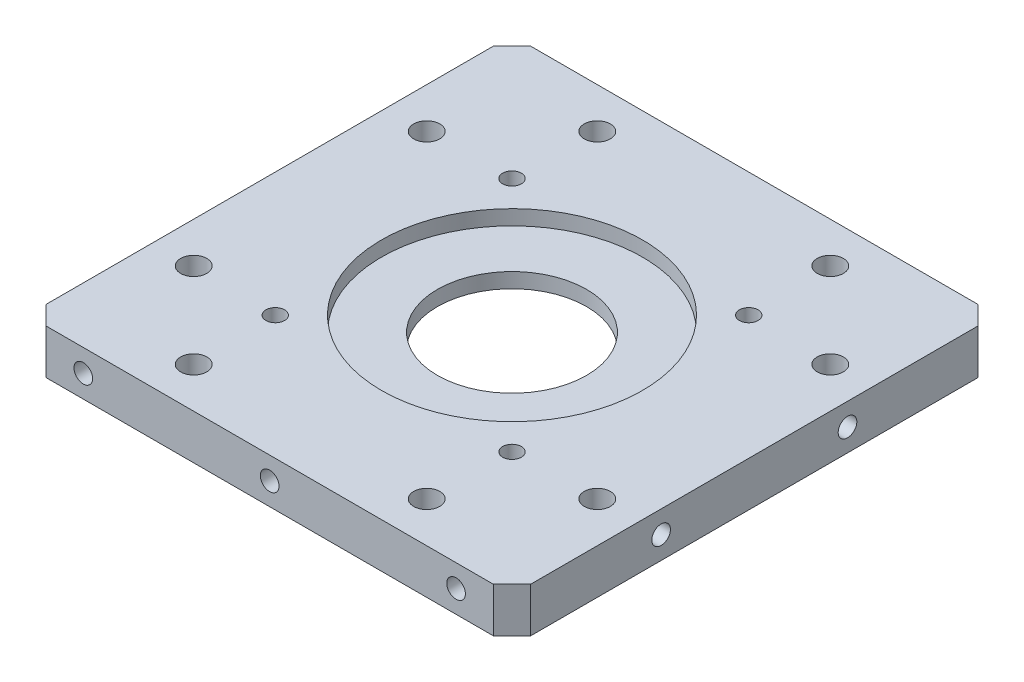
from build123d import *

# Parameters (mm, degrees)
SKETCH_1_W             = 130
SKETCH_1_H             = 130
EXTRUDE_1_DEPTH        = 12
SKETCH_2_R             = 20
CUT_EXTRUDE_1_DEPTH    = 93.703829479
HOLE_WIZARD_M6_1_D     = 7
SKETCH_5_R             = 35
CUT_EXTRUDE_2_DEPTH    = 4
SKETCH_6_R             = 45
CUT_EXTRUDE_3_DEPTH    = 4
HOLE_WIZARD_M6_1_2_D   = 5
HOLE_WIZARD_M6_2_D     = 5
HOLE_WIZARD_M6_2_DEPTH = 15
HOLE_WIZARD_M6_2_TIP   = 1.502151548
HOLE_WIZARD_M6_3_D     = 5
HOLE_WIZARD_M6_3_DEPTH = 15
HOLE_WIZARD_M6_3_TIP   = 1.502151548
HOLE_WIZARD_M6_4_D     = 5
HOLE_WIZARD_M6_4_DEPTH = 15
HOLE_WIZARD_M6_4_TIP   = 1.502151548
HOLE_WIZARD_M6_5_D     = 5
HOLE_WIZARD_M6_5_DEPTH = 15
HOLE_WIZARD_M6_5_TIP   = 1.502151548
CHAMFER_1_SIZE         = 5


with BuildPart() as part:
    # 草图1 → 凸台-拉伸1 (new body)
    with BuildSketch(Plane(origin=(0, 0, 0), x_dir=(1, 0, 0), z_dir=(0, 1, 0))):
        Rectangle(SKETCH_1_W, SKETCH_1_H)
    extrude(amount=EXTRUDE_1_DEPTH)

    # 草图2 → 切除-拉伸1 (cut, through all)
    with BuildSketch(Plane(origin=(0, 12, 0), x_dir=(1, 0, 0), z_dir=(0, 1, 0))):
        with Locations(Location((0, 0, 0), (0, 0, 270))):
            Circle(SKETCH_2_R)
    extrude(amount=-CUT_EXTRUDE_1_DEPTH, mode=Mode.SUBTRACT)

    # Hole Wizard M6 _1 (through all)
    with Locations(Plane(origin=(0, 12, 0), x_dir=(1, 0, 0), z_dir=(0, 1, 0))):
        with Locations((31.250000582, 54.1265874), (54.126588073, 31.249999418), (54.1265874, -31.250000582), (31.249999418, -54.126588073), (-31.250000582, -54.1265874), (-54.126588073, -31.249999418), (-54.1265874, 31.250000582), (-31.249999418, 54.126588073)):
            Hole(HOLE_WIZARD_M6_1_D / 2)

    # 草图5 → 切除-拉伸2 (cut)
    with BuildSketch(Plane(origin=(0, 12, 0), x_dir=(1, 0, 0), z_dir=(0, 1, 0))):
        with Locations(Location((0, 0, 0), (0, 0, 270))):
            Circle(SKETCH_5_R)
    extrude(amount=-CUT_EXTRUDE_2_DEPTH, mode=Mode.SUBTRACT)

    # 草图6 → 切除-拉伸3 (cut)
    with BuildSketch(Plane.XZ):
        with Locations(Location((0, 0, 0), (0, 0, 270))):
            Circle(SKETCH_6_R)
    extrude(amount=-CUT_EXTRUDE_3_DEPTH, mode=Mode.SUBTRACT)

    # Hole Wizard M6 _1 2 (through all)
    with Locations(Plane(origin=(0, 12, 0), x_dir=(1, 0, 0), z_dir=(0, 1, 0))):
        with Locations((-31.75, 31.75), (31.75, 31.75), (31.75, -31.75), (-31.75, -31.75)):
            Hole(HOLE_WIZARD_M6_1_2_D / 2)

    # M6 螺纹孔2
    with Locations(Plane.ZY.offset(65)):
        with Locations((-25, 6), (25, 6)):
            Hole(HOLE_WIZARD_M6_2_D / 2, depth=HOLE_WIZARD_M6_2_DEPTH)
            with Locations((0, 0, -(HOLE_WIZARD_M6_2_DEPTH + HOLE_WIZARD_M6_2_TIP / 2))):  # 118° drill point
                Cone(0, HOLE_WIZARD_M6_2_D / 2, HOLE_WIZARD_M6_2_TIP, mode=Mode.SUBTRACT)

    # M6 螺纹孔3
    with Locations(Plane(origin=(65, 0, 0), x_dir=(0, 0, -1), z_dir=(1, 0, 0))):
        with Locations((-25, 6), (25, 6)):
            Hole(HOLE_WIZARD_M6_3_D / 2, depth=HOLE_WIZARD_M6_3_DEPTH)
            with Locations((0, 0, -(HOLE_WIZARD_M6_3_DEPTH + HOLE_WIZARD_M6_3_TIP / 2))):  # 118° drill point
                Cone(0, HOLE_WIZARD_M6_3_D / 2, HOLE_WIZARD_M6_3_TIP, mode=Mode.SUBTRACT)

    # M6 螺纹孔4
    with Locations(Plane.XY.offset(65)):
        with Locations((-50, 6), (50, 6), (0, 6)):
            Hole(HOLE_WIZARD_M6_4_D / 2, depth=HOLE_WIZARD_M6_4_DEPTH)
            with Locations((0, 0, -(HOLE_WIZARD_M6_4_DEPTH + HOLE_WIZARD_M6_4_TIP / 2))):  # 118° drill point
                Cone(0, HOLE_WIZARD_M6_4_D / 2, HOLE_WIZARD_M6_4_TIP, mode=Mode.SUBTRACT)

    # M6 螺纹孔5
    with Locations(Plane(origin=(0, 0, -65), x_dir=(-1, 0, 0), z_dir=(0, 0, -1))):
        with Locations((-50, 6), (50, 6), (0, 6)):
            Hole(HOLE_WIZARD_M6_5_D / 2, depth=HOLE_WIZARD_M6_5_DEPTH)
            with Locations((0, 0, -(HOLE_WIZARD_M6_5_DEPTH + HOLE_WIZARD_M6_5_TIP / 2))):  # 118° drill point
                Cone(0, HOLE_WIZARD_M6_5_D / 2, HOLE_WIZARD_M6_5_TIP, mode=Mode.SUBTRACT)

    # 倒角1
    chamfer_1_edges = [part.edges().sort_by_distance(p)[0] for p in [
        (65, 6, 65),
        (-65, 6, 65),
        (-65, 6, -65),
        (65, 6, -65),
    ]]
    chamfer(chamfer_1_edges, length=CHAMFER_1_SIZE)


solid = part.part
